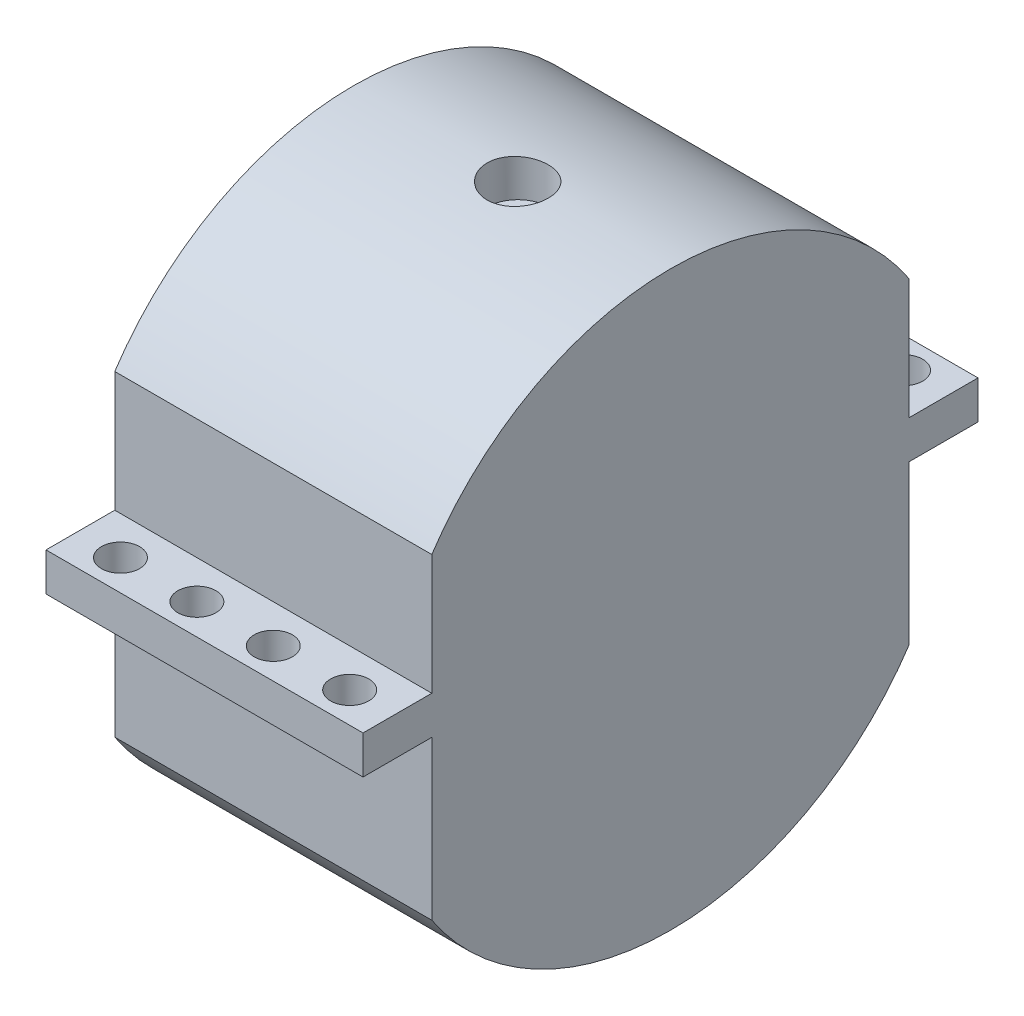
from build123d import *

# Parameters (mm, degrees)
CUT_EXTRUDE_1_REACH      = 136.681
SKETCH_9_W               = 18
SKETCH_9_H               = 10
EXTRUDE_1_DEPTH          = 83
CUT_EXTRUDE_4_REACH      = 165.25
SKETCH_10_R              = 5
CUT_EXTRUDE_5_REACH      = 206.757
CUT_EXTRUDE_5_END_RADIUS = 40
SKETCH_11_R              = 5
SKETCH_12_R              = 8
CUT_EXTRUDE_6_DEPTH      = 10


with BuildPart() as part:
    # 草图1 → 旋转1 (revolve)
    with BuildSketch(Plane.XY, mode=Mode.PRIVATE) as revolve_1_sk:
        Polygon((30.777777778, 50), (30.777777778, 75), (113.777777778, 75), (113.777777778, 0), (93.777777778, 0), (93.777777778, 30), (95.777777778, 32), (95.777777778, 40), (43.777777778, 40), (43.777777778, 50), align=None)
    revolve(revolve_1_sk.sketch.rotate(Axis((-130.37037037, 0, 0), (1, 0, 0)), 90), axis=Axis((-130.37037037, 0, 0), (1, 0, 0)))

    # 草图6 → 切除-拉伸1 (cut, up to next)
    with BuildSketch(Plane(origin=(113.777777778, 0, 0), x_dir=(0, 0, -1), z_dir=(1, 0, 0)), mode=Mode.PRIVATE) as cut_extrude_1_sk1:
        with BuildLine():
            Line((62.5, 41.457809879), (62.5, -41.457809879))
            ThreePointArc((62.5, -41.457809879), (75, 0), (62.5, 41.457809879))
        make_face()
    cut_extrude_1_tool1 = extrude(cut_extrude_1_sk1.sketch, amount=-CUT_EXTRUDE_1_REACH, mode=Mode.PRIVATE) & part.part
    # 草图6 → 切除-拉伸1 (cut, up to next)
    with BuildSketch(Plane(origin=(113.777777778, 0, 0), x_dir=(0, 0, -1), z_dir=(1, 0, 0)), mode=Mode.PRIVATE) as cut_extrude_1_sk2:
        with BuildLine():
            Line((-62.5, 41.457809879), (-62.5, -41.457809879))
            ThreePointArc((-62.5, -41.457809879), (-75, 0), (-62.5, 41.457809879))
        make_face()
    cut_extrude_1_tool2 = extrude(cut_extrude_1_sk2.sketch, amount=-CUT_EXTRUDE_1_REACH, mode=Mode.PRIVATE) & part.part
    add(cut_extrude_1_tool1.solids().sort_by_distance((113.777778, 0, -67.537528))[0], mode=Mode.SUBTRACT)
    add(cut_extrude_1_tool2.solids().sort_by_distance((113.777778, 0, 67.537528))[0], mode=Mode.SUBTRACT)

    # 草图9 → 凸台-拉伸1 (add)
    with BuildSketch(Plane(origin=(113.777777778, 0, 0), x_dir=(0, 0, -1), z_dir=(1, 0, 0))):
        with Locations((-71.5, 5)):
            Rectangle(SKETCH_9_W, SKETCH_9_H)
        with Locations((71.5, 5)):
            Rectangle(SKETCH_9_W, SKETCH_9_H)
    extrude(amount=-EXTRUDE_1_DEPTH)

    # 草图10 → 切除-拉伸4 (cut, up to next)
    with BuildSketch(Plane(origin=(0, 10, 0), x_dir=(1, 0, 0), z_dir=(0, 1, 0)), mode=Mode.PRIVATE) as cut_extrude_4_sk1:
        with Locations(Location((42.277777778, 72.5, 0), (0, 0, 270))):
            Circle(SKETCH_10_R)
    cut_extrude_4_tool1 = extrude(cut_extrude_4_sk1.sketch, amount=-CUT_EXTRUDE_4_REACH, mode=Mode.PRIVATE) & part.part
    # 草图10 → 切除-拉伸4 (cut, up to next)
    with BuildSketch(Plane(origin=(0, 10, 0), x_dir=(1, 0, 0), z_dir=(0, 1, 0)), mode=Mode.PRIVATE) as cut_extrude_4_sk2:
        with Locations(Location((62.277777778, 72.5, 0), (0, 0, 270))):
            Circle(SKETCH_10_R)
    cut_extrude_4_tool2 = extrude(cut_extrude_4_sk2.sketch, amount=-CUT_EXTRUDE_4_REACH, mode=Mode.PRIVATE) & part.part
    # 草图10 → 切除-拉伸4 (cut, up to next)
    with BuildSketch(Plane(origin=(0, 10, 0), x_dir=(1, 0, 0), z_dir=(0, 1, 0)), mode=Mode.PRIVATE) as cut_extrude_4_sk3:
        with Locations(Location((82.277777778, 72.5, 0), (0, 0, 270))):
            Circle(SKETCH_10_R)
    cut_extrude_4_tool3 = extrude(cut_extrude_4_sk3.sketch, amount=-CUT_EXTRUDE_4_REACH, mode=Mode.PRIVATE) & part.part
    # 草图10 → 切除-拉伸4 (cut, up to next)
    with BuildSketch(Plane(origin=(0, 10, 0), x_dir=(1, 0, 0), z_dir=(0, 1, 0)), mode=Mode.PRIVATE) as cut_extrude_4_sk4:
        with Locations(Location((102.277777778, 72.5, 0), (0, 0, 270))):
            Circle(SKETCH_10_R)
    cut_extrude_4_tool4 = extrude(cut_extrude_4_sk4.sketch, amount=-CUT_EXTRUDE_4_REACH, mode=Mode.PRIVATE) & part.part
    # 草图10 → 切除-拉伸4 (cut, up to next)
    with BuildSketch(Plane(origin=(0, 10, 0), x_dir=(1, 0, 0), z_dir=(0, 1, 0)), mode=Mode.PRIVATE) as cut_extrude_4_sk5:
        with Locations(Location((102.277777778, -72.5, 0), (0, 0, 90))):
            Circle(SKETCH_10_R)
    cut_extrude_4_tool5 = extrude(cut_extrude_4_sk5.sketch, amount=-CUT_EXTRUDE_4_REACH, mode=Mode.PRIVATE) & part.part
    # 草图10 → 切除-拉伸4 (cut, up to next)
    with BuildSketch(Plane(origin=(0, 10, 0), x_dir=(1, 0, 0), z_dir=(0, 1, 0)), mode=Mode.PRIVATE) as cut_extrude_4_sk6:
        with Locations(Location((82.277777778, -72.5, 0), (0, 0, 90))):
            Circle(SKETCH_10_R)
    cut_extrude_4_tool6 = extrude(cut_extrude_4_sk6.sketch, amount=-CUT_EXTRUDE_4_REACH, mode=Mode.PRIVATE) & part.part
    # 草图10 → 切除-拉伸4 (cut, up to next)
    with BuildSketch(Plane(origin=(0, 10, 0), x_dir=(1, 0, 0), z_dir=(0, 1, 0)), mode=Mode.PRIVATE) as cut_extrude_4_sk7:
        with Locations(Location((62.277777778, -72.5, 0), (0, 0, 90))):
            Circle(SKETCH_10_R)
    cut_extrude_4_tool7 = extrude(cut_extrude_4_sk7.sketch, amount=-CUT_EXTRUDE_4_REACH, mode=Mode.PRIVATE) & part.part
    # 草图10 → 切除-拉伸4 (cut, up to next)
    with BuildSketch(Plane(origin=(0, 10, 0), x_dir=(1, 0, 0), z_dir=(0, 1, 0)), mode=Mode.PRIVATE) as cut_extrude_4_sk8:
        with Locations(Location((42.277777778, -72.5, 0), (0, 0, 90))):
            Circle(SKETCH_10_R)
    cut_extrude_4_tool8 = extrude(cut_extrude_4_sk8.sketch, amount=-CUT_EXTRUDE_4_REACH, mode=Mode.PRIVATE) & part.part
    add(cut_extrude_4_tool1.solids().sort_by_distance((42.277778, 10, -72.5))[0], mode=Mode.SUBTRACT)
    add(cut_extrude_4_tool2.solids().sort_by_distance((62.277778, 10, -72.5))[0], mode=Mode.SUBTRACT)
    add(cut_extrude_4_tool3.solids().sort_by_distance((82.277778, 10, -72.5))[0], mode=Mode.SUBTRACT)
    add(cut_extrude_4_tool4.solids().sort_by_distance((102.277778, 10, -72.5))[0], mode=Mode.SUBTRACT)
    add(cut_extrude_4_tool5.solids().sort_by_distance((102.277778, 10, 72.5))[0], mode=Mode.SUBTRACT)
    add(cut_extrude_4_tool6.solids().sort_by_distance((82.277778, 10, 72.5))[0], mode=Mode.SUBTRACT)
    add(cut_extrude_4_tool7.solids().sort_by_distance((62.277778, 10, 72.5))[0], mode=Mode.SUBTRACT)
    add(cut_extrude_4_tool8.solids().sort_by_distance((42.277778, 10, 72.5))[0], mode=Mode.SUBTRACT)

    # 切除-拉伸5: up to this cylinder (the profile starts outside it)
    cut_extrude_5_end = Plane(origin=(73.777778, 0, 0), z_dir=(-1, 0, 0)) * Cylinder(CUT_EXTRUDE_5_END_RADIUS, 494.514, mode=Mode.PRIVATE)
    # 草图11 → 切除-拉伸5 (cut, up to the surface)
    with BuildSketch(Plane(origin=(0, 75, 0), x_dir=(1, 0, 0), z_dir=(0, 1, 0)), mode=Mode.PRIVATE) as cut_extrude_5_sk1:
        with Locations(Location((73.777777778, 0, 0), (0, 0, 270))):
            Circle(SKETCH_11_R)
    cut_extrude_5_tool1 = extrude(cut_extrude_5_sk1.sketch, amount=-CUT_EXTRUDE_5_REACH, mode=Mode.PRIVATE) - cut_extrude_5_end
    add(cut_extrude_5_tool1.solids().sort_by_distance((73.777778, 75, 0))[0], mode=Mode.SUBTRACT)

    # 草图12 → 切除-拉伸6 (cut)
    with BuildSketch(Plane(origin=(0, 75, 0), x_dir=(1, 0, 0), z_dir=(0, 1, 0))):
        with Locations(Location((73.777777778, 0, 0), (0, 0, 270))):
            Circle(SKETCH_12_R)
    extrude(amount=-CUT_EXTRUDE_6_DEPTH, mode=Mode.SUBTRACT)


solid = part.part
